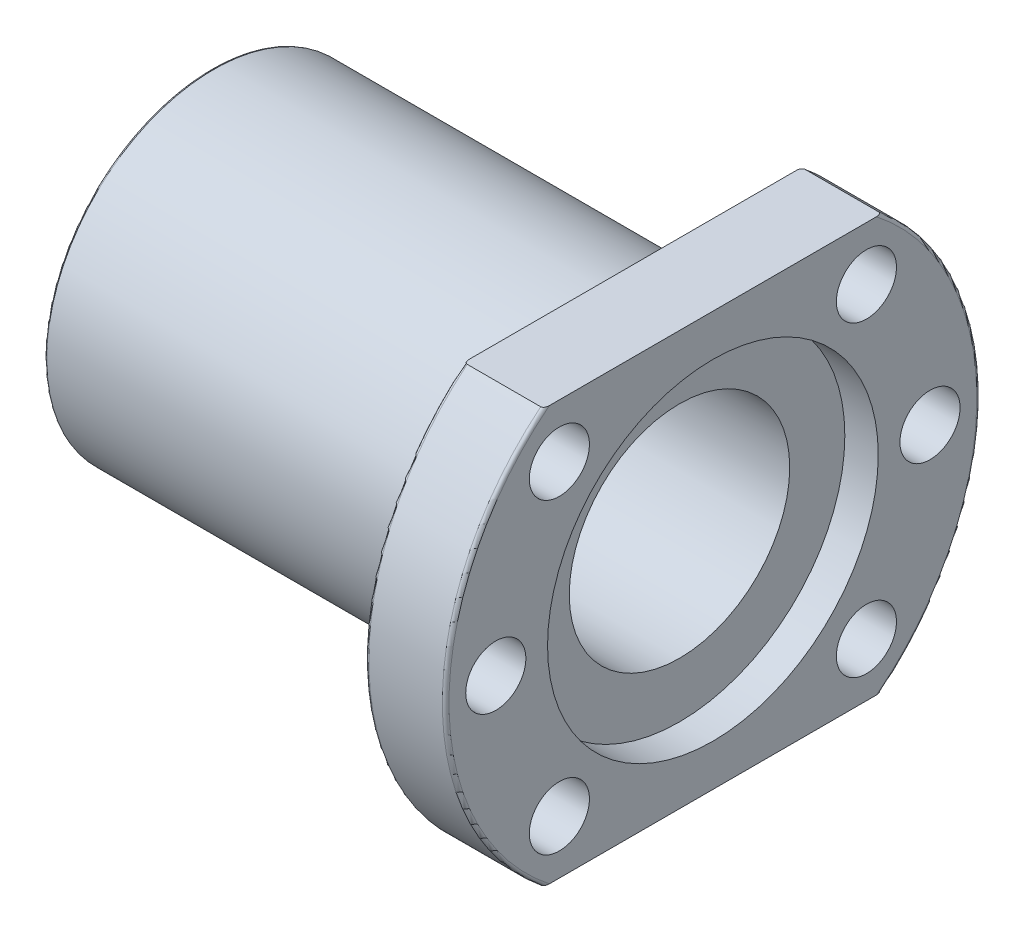
from build123d import *

# Parameters (mm, degrees)
EXTRUDE_1_DEPTH               = 11.999999998
SKETCH_2_W                    = 63.000000153
SKETCH_2_H                    = 24.999999254
HOLE_WIZARD_9_0_9_1_D         = 9
HOLE_WIZARD_M30_1_D           = 32.999998421
HOLE_WIZARD_M30_1_CBORE_D     = 49.499997436
HOLE_WIZARD_M30_1_CBORE_DEPTH = 5
FILLET_1_R                    = 0.3
FILLET_2_R                    = 0.5


with BuildPart() as part:
    # 草图1 → 凸台-拉伸1 (new body)
    with BuildSketch(Plane(origin=(-19.893035878, 0, 0), x_dir=(0, 0, -1), z_dir=(1, 0, 0))):
        with BuildLine():
            Line((25.278447364, 30.999999739), (-25.278447364, 30.999999739))
            ThreePointArc((-25.278447364, 30.999999739), (-39.999998764, -2.61e-07), (-25.278447364, -31.000000261))
            Line((-25.278447364, -31.000000261), (25.278447364, -31.000000261))
            ThreePointArc((25.278447364, -31.000000261), (39.999998764, -2.61e-07), (25.278447364, 30.999999739))
        make_face()
    extrude(amount=-EXTRUDE_1_DEPTH)

    # 草图2 → 旋转1 (revolve)
    with BuildSketch(Plane.XY, mode=Mode.PRIVATE) as revolve_1_sk:
        with Locations((-63.393035954, 12.499998381)):
            Rectangle(SKETCH_2_W, SKETCH_2_H)
    revolve(revolve_1_sk.sketch.rotate(Axis((-94.89303603, -1.246e-06, 0), (1, 0, 0)), 270), axis=Axis((-94.89303603, -1.246e-06, 0), (1, 0, 0)))

    # Ø9.0 (9) 直径孔1 (through all)
    with Locations(Plane.ZY.offset(31.893035877)):
        with Locations((22.981, 22.980999581), (22.981, -22.981000419), (-22.981, -22.981000419), (-22.981, 22.980999581), (32.5, -4.19e-07), (-32.5, -4.19e-07)):
            Hole(HOLE_WIZARD_9_0_9_1_D / 2)

    # M30 六角头螺栓的柱形沉头孔1 (through all)
    with Locations(Plane(origin=(-19.893035878, 0, 0), x_dir=(0, 0, -1), z_dir=(1, 0, 0))):
        with Locations((0, -2.61e-07)):
            CounterBoreHole(HOLE_WIZARD_M30_1_D / 2, HOLE_WIZARD_M30_1_CBORE_D / 2, HOLE_WIZARD_M30_1_CBORE_DEPTH)

    # 圆角1
    fillet_1_edges = [part.edges().sort_by_distance(p)[0] for p in [
        (-94.89303603, -1.246e-06, 24.999999255),
    ]]
    fillet(fillet_1_edges, radius=FILLET_1_R)

    # 圆角2
    fillet_2_edges = [part.edges().sort_by_distance(p)[0] for p in [
        (-31.893035877, -2.61e-07, 39.999998764),
        (-31.893035877, -2.61e-07, -39.999998764),
        (-19.893035878, -2.61e-07, 39.999998764),
        (-19.893035878, -2.61e-07, -39.999998764),
    ]]
    fillet(fillet_2_edges, radius=FILLET_2_R)


solid = part.part
